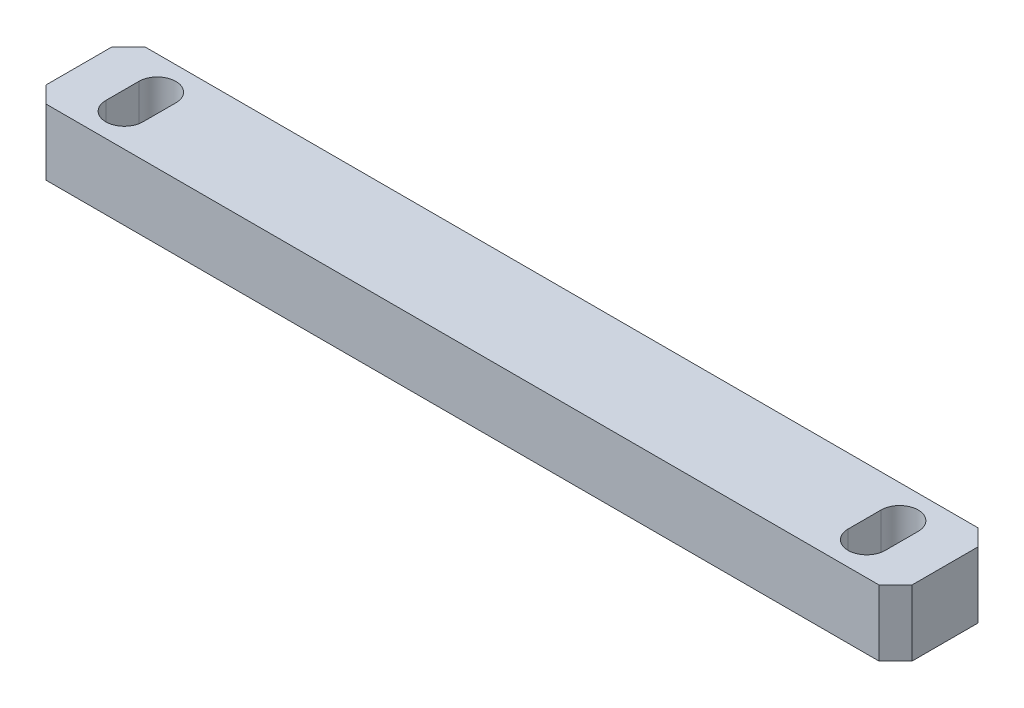
SolidWorks part; units mm, degrees
ref_plane "Front Plane" through (0, 0, 0) normal (0, 0, 1) x (1, 0, 0)
ref_plane "Top Plane" through (0, 0, 0) normal (0, 1, 0) x (1, 0, 0)
ref_plane "Right Plane" through (0, 0, 0) normal (1, 0, 0) x (0, 0, -1)
sketch "Sketch1" plane through (0, 0, 0) normal (0, 1, 0) x (1, 0, 0)
  line L1 (0, 0) -> (105, 0)
  line L2 (0, 0) -> (0, 12)
  line L3 (0, 12) -> (105, 12)
  line L4 (105, 0) -> (105, 12)
  dimension "D1" = 12
  dimension "D2" = 105
extrude "Boss-Extrude1" add sketch "Sketch1" along normal blind 8
chamfer "Chamfer1" distance 2 angle 45 4 edges at (105, 4, 0) (105, 4, -12) (0, 4, 0) (0, 4, -12)
sketch "Sketch2" plane through (0, 8, 0) normal (0, 1, 0) x (1, 0, 0)
  line L0 (52.5, 0) -> (52.5, 50000) construction
  line L1 (2, 0) -> (103, 0) construction
  line L2 (0, 6) -> (50000, 6) construction
  line L3 (0, 10) -> (0, 2) construction
  circle A0 centre (7.5, 6) radius 2.25
  circle A1 centre (97.5, 6) radius 2.25
  point P4 (52.5, 0)
  point P9 (0, 6)
  dimension "D1" = 4.5
  dimension "D2" = 90
extrude "Cut-Extrude1" cut sketch "Sketch2" against normal blind 10
sketch "Sketch3" plane through (0, 8, 0) normal (0, 1, 0) x (1, 0, 0)
  line L0 (7.5, 4) -> (7.5, 8) construction
  line L1 (5.25, 4) -> (5.25, 8)
  line L2 (9.75, 4) -> (9.75, 8)
  line L3 (52.5, 12) -> (52.5, -49988) construction
  line L4 (103, 12) -> (2, 12) construction
  line L5 (97.5, 4) -> (97.5, 8) construction
  line L6 (99.75, 4) -> (99.75, 8)
  line L7 (95.25, 4) -> (95.25, 8)
  arc A0 (5.25, 4) -> (9.75, 4) centre (7.5, 4) ccw
  arc A1 (9.75, 8) -> (5.25, 8) centre (7.5, 8) ccw
  arc A2 (99.75, 4) -> (95.25, 4) centre (97.5, 4) cw
  arc A3 (95.25, 8) -> (99.75, 8) centre (97.5, 8) cw
  point P2 (7.5, 6)
  point P12 (52.5, 12)
  point P15 (97.5, 6)
  dimension "D1" = 4.5
  dimension "D2" = 4
extrude "Cut-Extrude2" cut sketch "Sketch3" against normal blind 10
